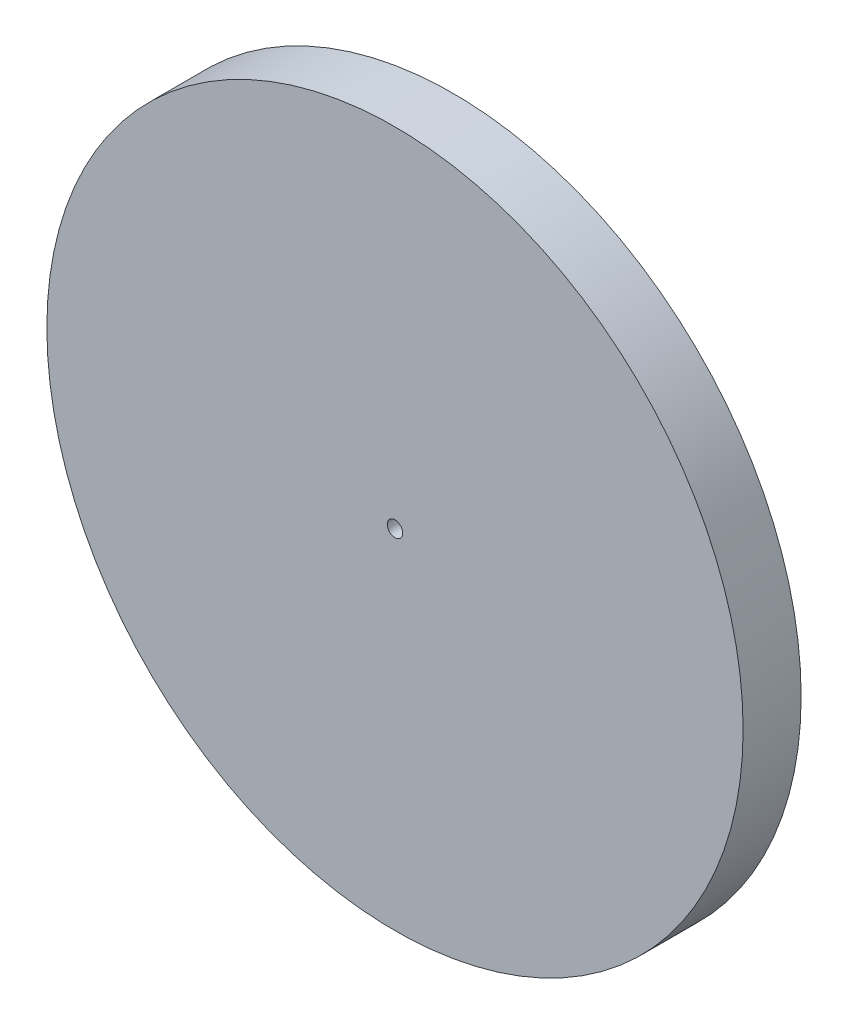
SolidWorks part; units mm, degrees
ref_plane "Front" through (0, 0, 0) normal (0, 0, 1) x (1, 0, 0)
ref_plane "Top" through (0, 0, 0) normal (0, 1, 0) x (1, 0, 0)
ref_plane "Right" through (0, 0, 0) normal (1, 0, 0) x (0, 0, -1)
sketch "Sketch1" plane through (0, 0, 0) normal (0, 0, 1) x (1, 0, 0)
  circle A0 centre (0, 0) radius 900
  dimension "D1" = 1800
extrude "Boss-Extrude1" add sketch "Sketch1" along normal blind 150
sketch "Sketch2" plane through (0, 0, 0) normal (0, 0, -1) x (-1, 0, 0)
  circle A0 centre (0, 0) radius 20
  dimension "D1" = 40
extrude "Cut-Extrude1" cut sketch "Sketch2" against normal through all
